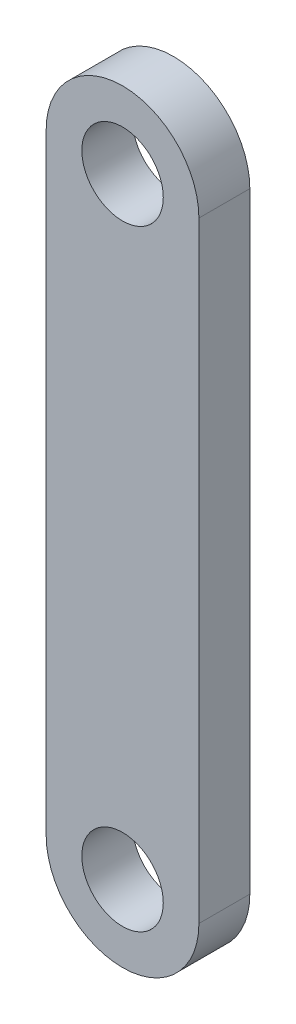
from build123d import *

# Parameters (mm, degrees)
SKETCH1_R           = 8
BOSS_EXTRUDE1_DEPTH = 10


with BuildPart() as part:
    # Sketch1 → Boss-Extrude1 (new body)
    with BuildSketch(Plane.XY):
        with BuildLine():
            Line((-15, 60), (-15, -60))
            ThreePointArc((-15, -60), (0, -75), (15, -60))
            Line((15, -60), (15, 60))
            ThreePointArc((15, 60), (0, 75), (-15, 60))
        make_face()
        with Locations((0, 60)):
            Circle(SKETCH1_R, mode=Mode.SUBTRACT)
        with Locations((0, -60)):
            Circle(SKETCH1_R, mode=Mode.SUBTRACT)
    extrude(amount=BOSS_EXTRUDE1_DEPTH)


solid = part.part
